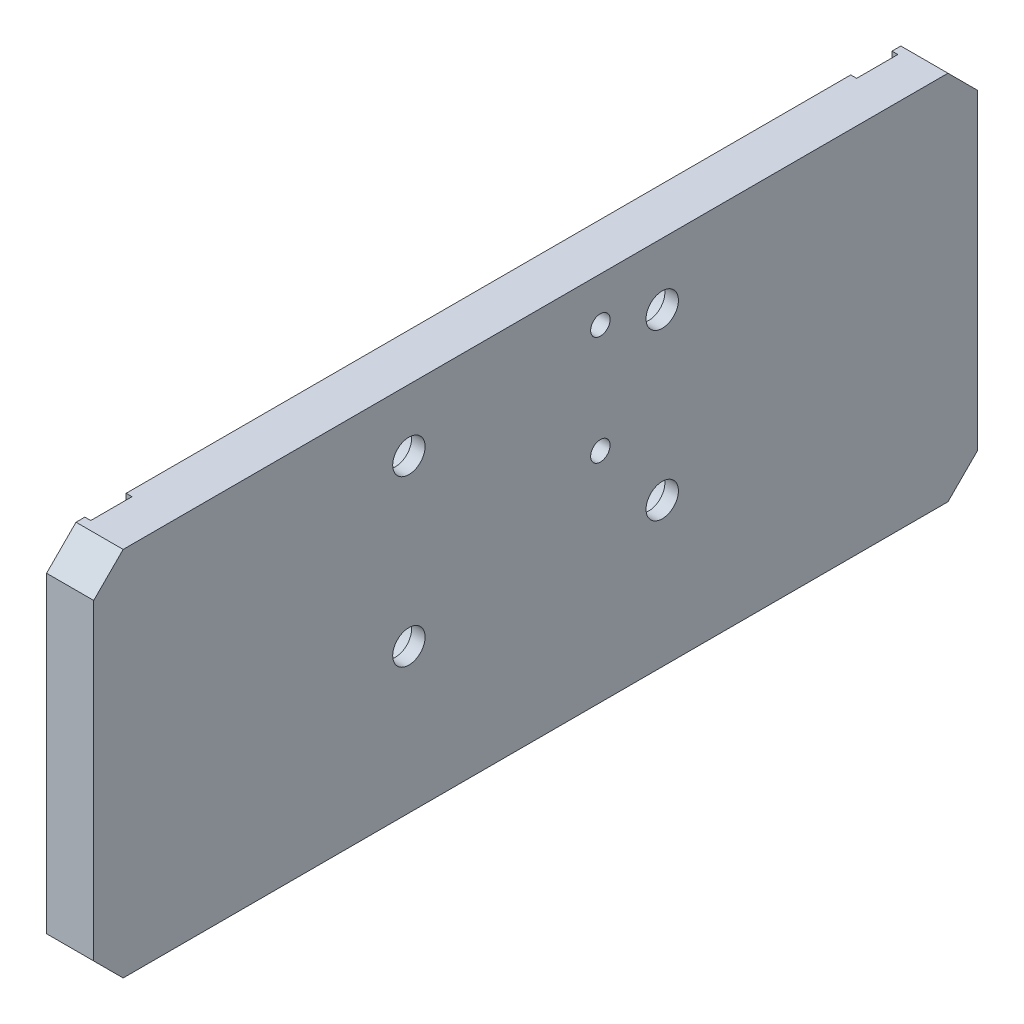
from build123d import *

# Parameters (mm, degrees)
SKETCH1_W                                    = 150
SKETCH1_H                                    = 63
BOSS_EXTRUDE1_DEPTH                          = 8
M4_TAPPED_HOLE1_D                            = 3.3
M4_TAPPED_HOLE1_DEPTH                        = 10.1
M4_TAPPED_HOLE1_TIP                          = 0.991420021
CBORE_FOR_M5_HEXAGON_SOCKET_HEAD_CAP_2_COUNT = 2
CBORE_FOR_M5_HEXAGON_SOCKET_HEAD_CAP_2_PITCH = 28
CBORE_FOR_M5_HEXAGON_SOCKET_HEAD_CAP_3_COUNT = 2
CBORE_FOR_M5_HEXAGON_SOCKET_HEAD_CAP_3_PITCH = 43
CBORE_FOR_M5_HEXAGON_SOCKET_HEAD_CAP_4_COUNT = 2
CBORE_FOR_M5_HEXAGON_SOCKET_HEAD_CAP_4_PITCH = 51.312766443
M2_TAPPED_HOLE1_D                            = 1.6
M2_TAPPED_HOLE1_DEPTH                        = 6.2
M2_TAPPED_HOLE1_TIP                          = 0.480688495
SKETCH17_W                                   = 7
SKETCH17_H                                   = 63
CUT_EXTRUDE1_DEPTH                           = 1
CHAMFER1_SIZE                                = 5


with BuildPart() as part:
    # Sketch1 → Boss-Extrude1 (new body)
    with BuildSketch(Plane(origin=(0, 0, 0), x_dir=(0, 0, -1), z_dir=(1, 0, 0))):
        Rectangle(SKETCH1_W, SKETCH1_H)
    extrude(amount=BOSS_EXTRUDE1_DEPTH)

    # M4 Tapped Hole1
    with Locations(Plane.ZY):
        with Locations((-11, 24), (-11, 5.5)):
            Hole(M4_TAPPED_HOLE1_D / 2, depth=M4_TAPPED_HOLE1_DEPTH)
            with Locations((0, 0, -(M4_TAPPED_HOLE1_DEPTH + M4_TAPPED_HOLE1_TIP / 2))):  # 118° drill point
                Cone(0, M4_TAPPED_HOLE1_D / 2, M4_TAPPED_HOLE1_TIP, mode=Mode.SUBTRACT)

    # Sketch15 → CBORE for M5 Hexagon socket head cap screws1 (revolve, cut)
    with BuildSketch(Plane(origin=(0, 21, 21.5), x_dir=(0, 0, 1), z_dir=(0, 1, 0))):
        Polygon((0, 0), (0, 14.052366702), (2.75, 12.4), (2.75, 5.7), (5, 5.7), (5, 0.025), (5.025, 0), align=None)
    cbore_for_m5_hexagon_socket_head_cap_scr = revolve(axis=Axis((-6.35, 21, 21.5), (1, 0, 0)), mode=Mode.SUBTRACT)

    # CBORE for M5 Hexagon socket head cap 2: CBORE for M5 Hexagon socket head cap screws1 ×2
    with Locations(*[(0, -i * CBORE_FOR_M5_HEXAGON_SOCKET_HEAD_CAP_2_PITCH, 0) for i in range(1, CBORE_FOR_M5_HEXAGON_SOCKET_HEAD_CAP_2_COUNT)]):
        add(cbore_for_m5_hexagon_socket_head_cap_scr, mode=Mode.SUBTRACT)

    # CBORE for M5 Hexagon socket head cap 3: CBORE for M5 Hexagon socket head cap screws1 ×2
    with Locations(*[(0, 0, -i * CBORE_FOR_M5_HEXAGON_SOCKET_HEAD_CAP_3_PITCH) for i in range(1, CBORE_FOR_M5_HEXAGON_SOCKET_HEAD_CAP_3_COUNT)]):
        add(cbore_for_m5_hexagon_socket_head_cap_scr, mode=Mode.SUBTRACT)

    # CBORE for M5 Hexagon socket head cap 4: CBORE for M5 Hexagon socket head cap screws1 ×2
    with Locations(*[Vector(0, -0.5456731714374324, -0.8379980847074858) * (i * CBORE_FOR_M5_HEXAGON_SOCKET_HEAD_CAP_4_PITCH) for i in range(1, CBORE_FOR_M5_HEXAGON_SOCKET_HEAD_CAP_4_COUNT)]):
        add(cbore_for_m5_hexagon_socket_head_cap_scr, mode=Mode.SUBTRACT)

    # M2 Tapped Hole1
    with Locations(Plane.ZY):
        with Locations((-65, 18.5), (-65, 3.5), (-65, -11.5), (65, -11.5), (65, 3.5), (65, 18.5)):
            Hole(M2_TAPPED_HOLE1_D / 2, depth=M2_TAPPED_HOLE1_DEPTH)
            with Locations((0, 0, -(M2_TAPPED_HOLE1_DEPTH + M2_TAPPED_HOLE1_TIP / 2))):  # 118° drill point
                Cone(0, M2_TAPPED_HOLE1_D / 2, M2_TAPPED_HOLE1_TIP, mode=Mode.SUBTRACT)

    # Sketch17 → Cut-Extrude1 (cut)
    with BuildSketch(Plane.ZY):
        with Locations((65, 0)):
            Rectangle(SKETCH17_W, SKETCH17_H)
        with Locations((-65, 0)):
            Rectangle(SKETCH17_W, SKETCH17_H)
    extrude(amount=-CUT_EXTRUDE1_DEPTH, mode=Mode.SUBTRACT)

    # Chamfer1
    chamfer1_edges = [part.edges().sort_by_distance(p)[0] for p in [
        (4, -31.5, -75),
        (4, -31.5, 75),
        (4, 31.5, 75),
        (4, 31.5, -75),
    ]]
    chamfer(chamfer1_edges, length=CHAMFER1_SIZE)


solid = part.part
